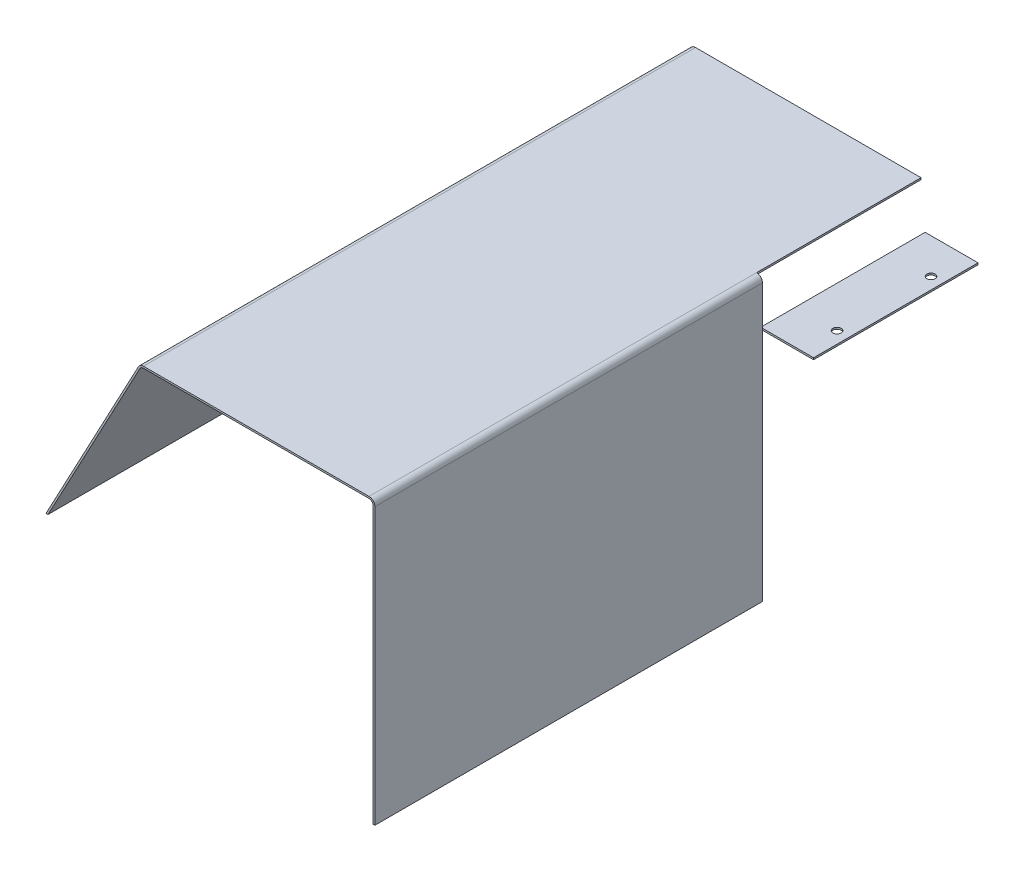
SolidWorks part; units mm, degrees
material "1023 Carbon Steel Plate (SS)"
ref_plane "Front Plane" through (0, 0, 0) normal (0, 0, 1) x (1, 0, 0)
ref_plane "Top Plane" through (0, 0, 0) normal (0, 1, 0) x (1, 0, 0)
ref_plane "Right Plane" through (0, 0, 0) normal (1, 0, 0) x (0, 0, -1)
sketch "Sketch1" plane through (0, 0, 0) normal (0, 0, 1) x (1, 0, 0)
  line L0 (0, 0) -> (78.5882, 147.3529)
  line L1 (83, 150) -> (275, 150)
  line L2 (280, 145) -> (280, -90)
  line L3 (1.7, 0) -> (79.9118, 146.6471)
  line L4 (83, 148.5) -> (275, 148.5)
  line L5 (278.5, 145) -> (278.5, -90)
  line L6 (0, 0) -> (1.7, 0)
  line L7 (280, -90) -> (278.5, -90)
  line L9 (1.3235, -0.7059) -> (79.9118, 146.6471) construction
  arc A0 (280, 145) -> (275, 150) centre (275, 145) ccw
  arc A1 (78.5882, 147.3529) -> (83, 150) centre (83, 145) cw
  arc A2 (79.9118, 146.6471) -> (83, 148.5) centre (83, 145) cw
  arc A3 (278.5, 145) -> (275, 148.5) centre (275, 145) ccw
  point P7 (280, 150)
  point P10 (80, 150)
  dimension "D5" = 5
  dimension "D1" = 150
  dimension "D2" = 200
  dimension "D3" = 80
  dimension "D4" = 240
  dimension "D6" = 1.5
extrude "Boss-Extrude1" add sketch "Sketch1" along normal blind 470 contours L3 A2 L4 A3 L5 L7 L2 A0 L1 A1 L0 L6
sketch "Sketch2" plane through (278.5, 0, 0) normal (-1, 0, 0) x (0, 0, 1)
  line L0 (-119.3847, 145) -> (140, 145)
  line L1 (140, 145) -> (140, -169.4685)
  line L2 (140, -169.4685) -> (-119.3847, -169.4685)
  line L3 (-119.3847, -169.4685) -> (-119.3847, 145)
  line L4 (470, 150) -> (0, 150) construction
  line L6 (0, 0) -> (0, 147.3529) construction
  dimension "D1" = 5
  dimension "D2" = 140
ref_plane "Plane1" through (0, 110, 0) normal (0, 1, 0) x (1, 0, 0)
extrude "Cut-Extrude3" cut sketch "Sketch2" against normal blind 1.5 contours L3 L0 L1 L2
sketch "Sketch5" plane through (0, 150, 0) normal (0, 1, 0) x (1, 0, 0)
  line L0 (275, 0) -> (275, -140)
  line L1 (275, -470) -> (275, 0) construction
  line L2 (275, -140) -> (332.9282, -140)
  line L3 (332.9282, -140) -> (332.9282, 0)
  line L4 (332.9282, 0) -> (275, 0)
  dimension "D1" = 140
extrude "Cut-Extrude9" cut sketch "Sketch5" against normal blind 58.5
sketch "Sketch7" plane through (0, 110, 0) normal (0, 1, 0) x (1, 0, 0)
  line L0 (275, -140) -> (323.5, -140)
  line L1 (323.5, -140) -> (323.5, 0)
  line L2 (323.5, 0) -> (275, 0)
  line L3 (275, 0) -> (275, -140)
  dimension "D1" = 48.5
extrude "Boss-Extrude3" add sketch "Sketch7" along normal blind 1.5
other "Move Face1" face at (275, 110.75, 70) parameters "D1"=3.5
sketch "Sketch9" plane through (0, 111.5, 0) normal (0, 1, 0) x (1, 0, 0)
  line L0 (280, -140) -> (323.5, -140) construction
  line L1 (323.5, -140) -> (323.5, 0) construction
  circle A0 centre (313.5, -30) radius 3.5
  circle A1 centre (313.5, -110) radius 3.5
  dimension "D4" = 7
  dimension "D1" = 80
  dimension "D2" = 30
  dimension "D3" = 10
extrude "Cut-Extrude10" cut sketch "Sketch9" against normal blind 1.5
